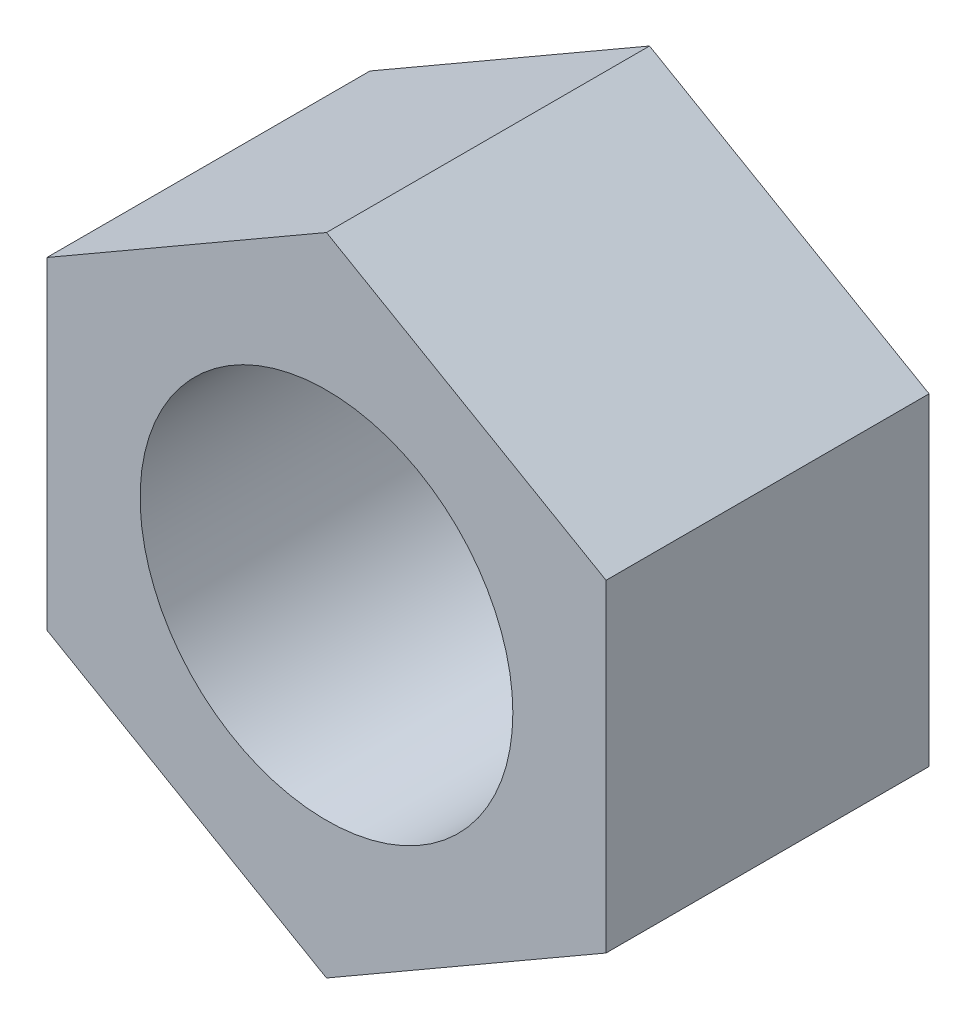
from build123d import *

# Parameters (mm, degrees)
SKETCH1_R           = 6
BOSS_EXTRUDE1_DEPTH = 10.4


with BuildPart() as part:
    # Sketch1 → Boss-Extrude1 (new body)
    with BuildSketch(Plane.XY):
        Polygon((0, -10.392304845), (9, -5.196152423), (9, 5.196152423), (0, 10.392304845), (-9, 5.196152423), (-9, -5.196152423), align=None)
        Circle(SKETCH1_R, mode=Mode.SUBTRACT)
    extrude(amount=BOSS_EXTRUDE1_DEPTH)


solid = part.part
